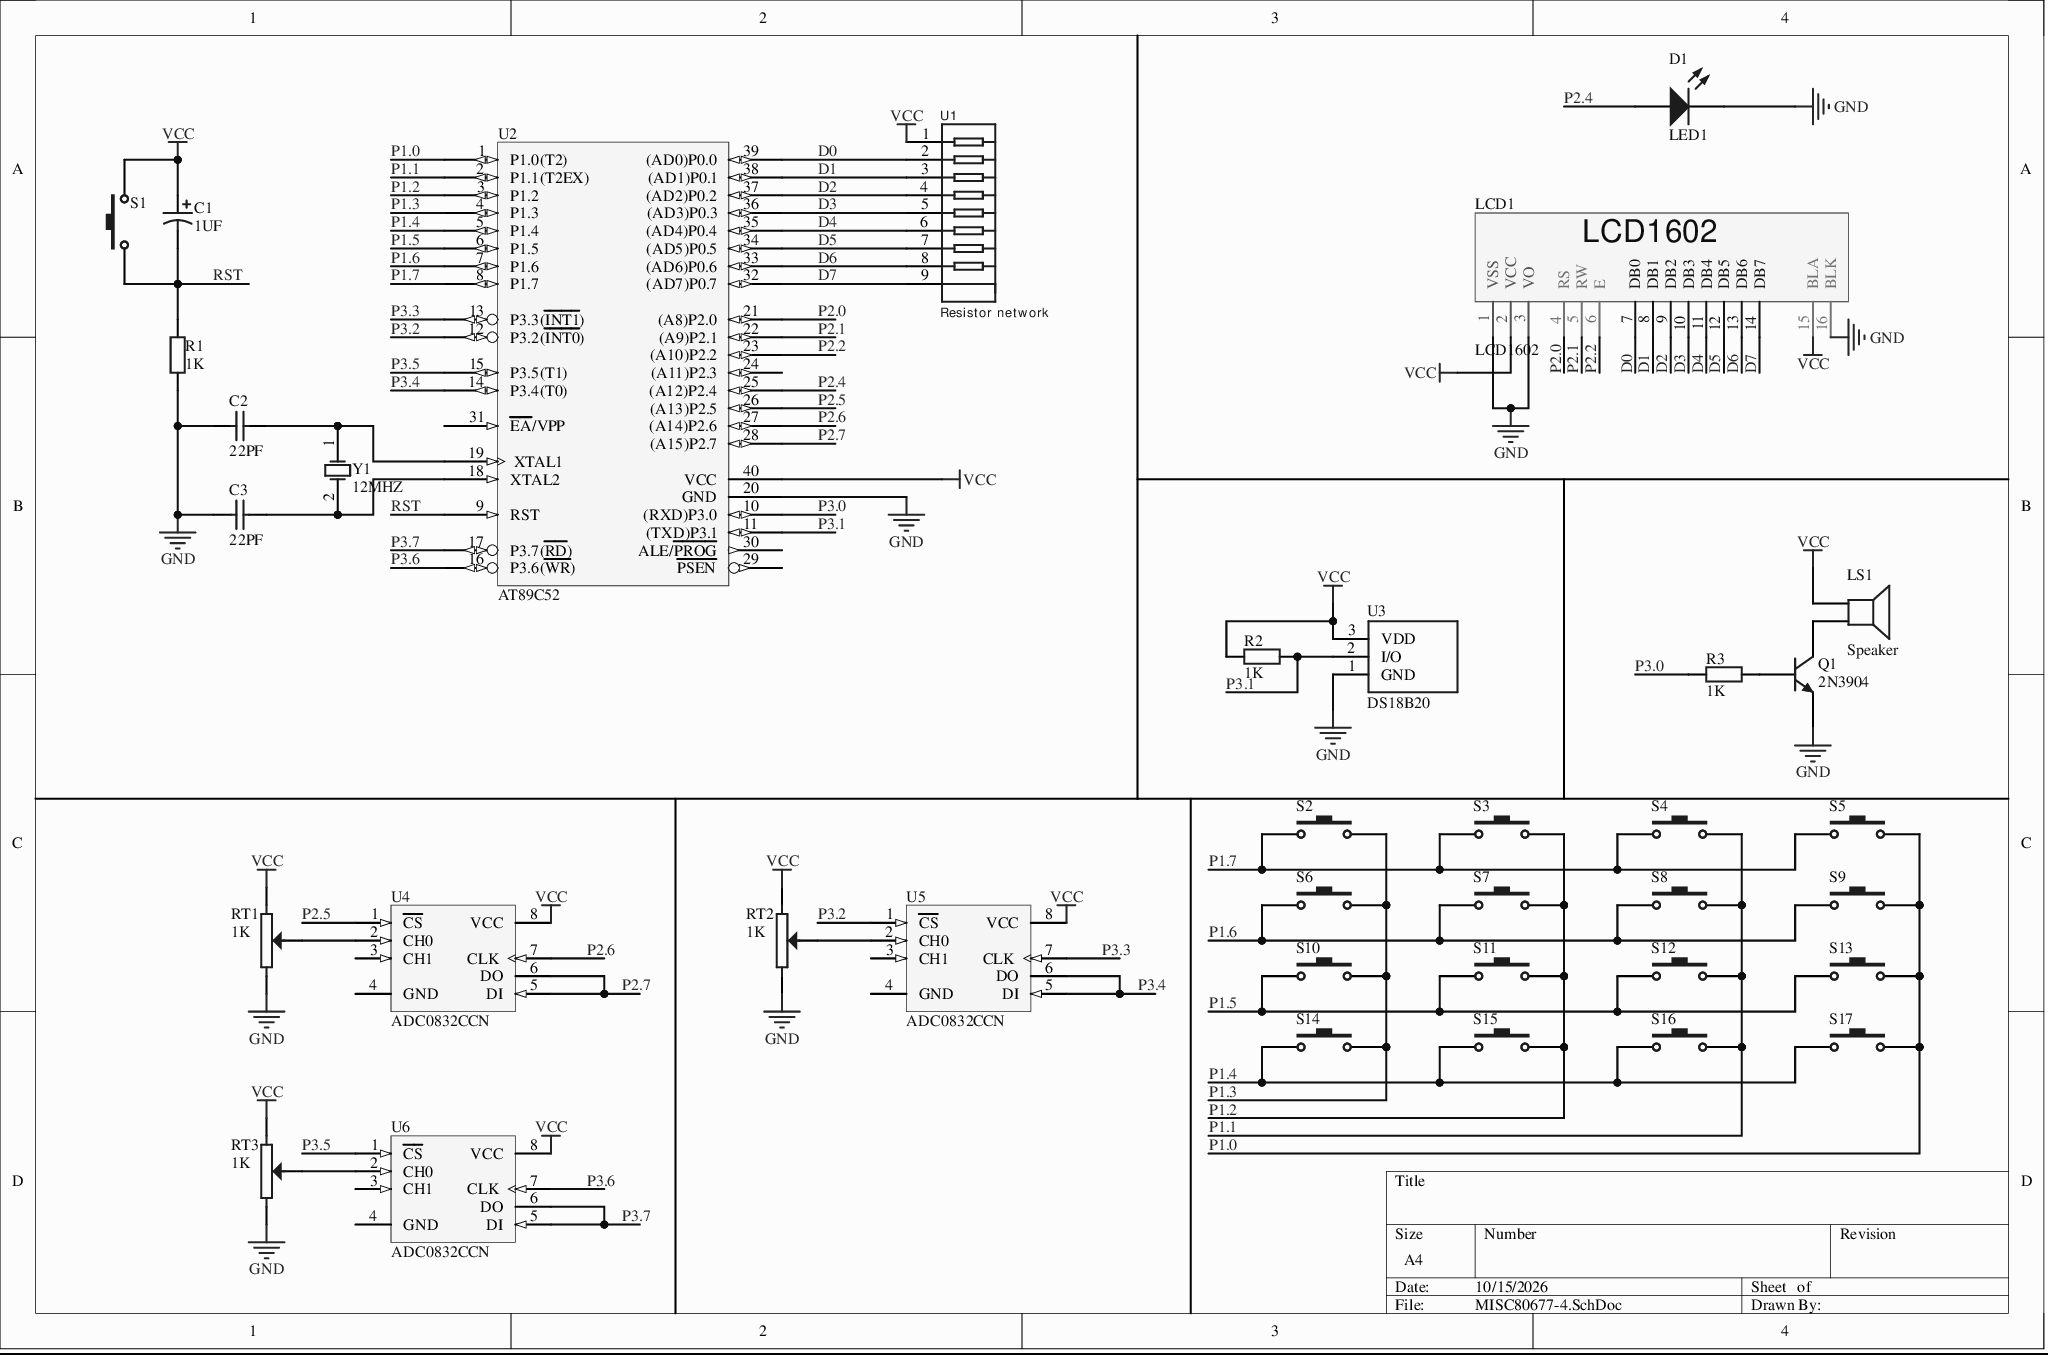
[diagram p0: MISC80677-4.SchDoc]
# Altium project MISC80677-7.PrjPcb
1 sheet, 37 parts. Net scope: global (net labels, ports and power ports of the same name join across sheets).
Board file: MISC80677.PcbDoc

## Sheet MISC80677-4.SchDoc
size A4

### Parts
C1  1UF  [RB7.6-15]
C2  22PF  [RAD-0.3]
C3  22PF  [RAD-0.3]
D1  LED1  [LED-1]
LCD1  LCD1602  [LCD1602]
LS1  Speaker  [PIN2]
Q1  2N3904  [TO-92A]
R1  1K  [AXIAL-0.4]
R2  1K  [AXIAL-0.4]
R3  1K  [AXIAL-0.4]
RT1  1K  [电位器]
RT2  1K  [电位器]
RT3  1K  [电位器]
S1  SW-PB  [SPST-2]  (value not drawn)
S2  SW-PB  [SPST-2]  (value not drawn)
S3  SW-PB  [SPST-2]  (value not drawn)
S4  SW-PB  [SPST-2]  (value not drawn)
S5  SW-PB  [SPST-2]  (value not drawn)
S6  SW-PB  [SPST-2]  (value not drawn)
S7  SW-PB  [SPST-2]  (value not drawn)
S8  SW-PB  [SPST-2]  (value not drawn)
S9  SW-PB  [SPST-2]  (value not drawn)
S10  SW-PB  [SPST-2]  (value not drawn)
S11  SW-PB  [SPST-2]  (value not drawn)
S12  SW-PB  [SPST-2]  (value not drawn)
S13  SW-PB  [SPST-2]  (value not drawn)
S14  SW-PB  [SPST-2]  (value not drawn)
S15  SW-PB  [SPST-2]  (value not drawn)
S16  SW-PB  [SPST-2]  (value not drawn)
S17  SW-PB  [SPST-2]  (value not drawn)
U1  Resistor network  [paizu]
U2  AT89C52  [DIP40]
U3  DS18B20  [DS18B20]
U4  ADC0832CCN  [N08E]
U5  ADC0832CCN  [N08E]
U6  ADC0832CCN  [N08E]
Y1  12MHZ  [R38]

### Nets
GND: C2.1 C3.1 D1.2(K) LCD1.1(VSS) LCD1.3(VO) LCD1.16(BLK) Q1.1(E) R1.1 RT1.2 RT2.2 RT3.2 U2.20(GND) U3.1(GND)
VCC: C1.1 LCD1.2(VCC) LCD1.15(BLA) LS1.1 R2.1 RT1.1 RT2.1 RT3.1 S1.2 U1.1 U2.40(VCC) U3.3(VDD) U4.8(VCC) U5.8(VCC) U6.8(VCC)
D0: LCD1.7(DB0) U1.2 U2.39((AD0)P0.0)
D1: LCD1.8(DB1) U1.3 U2.38((AD1)P0.1)
D2: LCD1.9(DB2) U1.4 U2.37((AD2)P0.2)
D3: LCD1.10(DB3) U1.5 U2.36((AD3)P0.3)
D4: LCD1.11(DB4) U1.6 U2.35((AD4)P0.4)
D5: LCD1.12(DB5) U1.7 U2.34((AD5)P0.5)
D6: LCD1.13(DB6) U1.8 U2.33((AD6)P0.6)
D7: LCD1.14(DB7) U1.9 U2.32((AD7)P0.7)
P1.0: S5.2 S9.2 S13.2 S17.2 U2.1(P1.0(T2))
P1.1: S4.2 S8.2 S12.2 S16.2 U2.2(P1.1(T2EX))
P1.2: S3.2 S7.2 S11.2 S15.2 U2.3(P1.2)
P1.3: S2.2 S6.2 S10.2 S14.2 U2.4(P1.3)
P1.4: S14.1 S15.1 S16.1 S17.1 U2.5(P1.4)
P1.5: S10.1 S11.1 S12.1 S13.1 U2.6(P1.5)
P1.6: S6.1 S7.1 S8.1 S9.1 U2.7(P1.6)
P1.7: S2.1 S3.1 S4.1 S5.1 U2.8(P1.7)
P2.0: LCD1.4(RS) U2.21((A8)P2.0)
P2.1: LCD1.5(RW) U2.22((A9)P2.1)
P2.2: LCD1.6(E) U2.23((A10)P2.2)
P2.4: D1.1(A) U2.25((A12)P2.4)
P2.5: U2.26((A13)P2.5) U4.1(~{CS})
P2.6: U2.27((A14)P2.6) U4.7(CLK)
P2.7: U2.28((A15)P2.7) U4.5(DI) U4.6(DO)
P3.0: R3.1 U2.10((RXD)P3.0)
P3.1: R2.2 U2.11((TXD)P3.1) U3.2(I/O)
P3.2: U2.12(P3.2(~{INT0})) U5.1(~{CS})
P3.3: U2.13(P3.3(~{INT1})) U5.7(CLK)
P3.4: U2.14(P3.4(T0)) U5.5(DI) U5.6(DO)
P3.5: U2.15(P3.5(T1)) U6.1(~{CS})
P3.6: U2.16(P3.6(~{WR})) U6.7(CLK)
P3.7: U2.17(P3.7(~{RD})) U6.5(DI) U6.6(DO)
RST: C1.2 R1.2 S1.1 U2.9(RST)
NetC2_2: C2.2 U2.19(XTAL1) Y1.1(OSC1)
NetC3_2: C3.2 U2.18(XTAL2) Y1.2(OSC2)
NetLS1_2: LS1.2 Q1.3(C)
NetQ1_2: Q1.2(B) R3.2
NetRT1_3: RT1.3(W) U4.2(CH0)
NetRT2_3: RT2.3(W) U5.2(CH0)
NetRT3_3: RT3.3(W) U6.2(CH0)

Not connected (* = marked no-connect by the designer): U2 24((A11)P2.3) 29(~{PSEN}) 30(ALE/~{PROG}) 31(~{EA}/VPP); U4 3(CH1) 4(GND); U5 3(CH1) 4(GND); U6 3(CH1) 4(GND)

### Library data of the parts
C1 = Cap Pol1: Polarized Capacitor (Radial); Value: 100pF; Published: 8-Jun-2000; LatestRevisionDate: 17-Jul-2002; LatestRevisionNote: Re-released for DXP Platform.; PackageReference: RB7.6-15; PackageDescription: Polarized Capacitor (Radial); 2 Leads; Publisher: Altium Limited
C2 C3 = Cap: Capacitor; Value: 100pF; Published: 8-Jun-2000; LatestRevisionDate: 17-Jul-2002; LatestRevisionNote: Re-released for DXP Platform.; PackageReference: RAD-0.3; PackageDescription: Radial Cap, Thru-Hole; 2 Leads; 0.3 in Pin Spacing; Publisher: Altium Limited
D1 = LED1: Typical RED GaAs LED; Published: 8-Jun-2000; LatestRevisionDate: 08-Jul-2005; LatestRevisionNote: Mech Layer 1 removed.; PackageReference: LED-1; PackageDescription: LED; 2 Leads; Publisher: Altium Limited
LS1 = Speaker: Loudspeaker; Published: 24-Mar-1999; LatestRevisionDate: 17-Jul-2002; LatestRevisionNote: Re-released for DXP Platform.; PackageReference: PIN2; Publisher: Altium Limited
Q1 = 2N3904: NPN General Purpose Amplifier; Published: 8-Jun-2000; LatestRevisionDate: 15-Jan-2003; LatestRevisionNote: PCB Footprint 'BCY-W3/D4.7' replaced; DatasheetVersion: 1997; PackageVersion: Sep-1998; PackageReference: TO-92A; PackageDescription: TO, Flat Index; 3 In-Line, Axial Leads; Body Dia. 4.5mm; Leads 0.51 x 0.48 mm (max); ComponentLink1Description: Manufacturer Link; ComponentLink2Description: Datasheet; ComponentLink2URL: http://www.fairchildsemi.com/ds/2N%2F2N3904.pdf; Publisher: Altium Limited
R1-R3 = Res2: Resistor; Published: 8-Jun-2000; LatestRevisionDate: 17-Jul-2002; LatestRevisionNote: Re-released for DXP Platform.; PackageReference: AXIAL-0.4; PackageDescription: Axial Device, Thru-Hole; 2 Leads; 0.4 in Pin Spacing; Value: 1K; Publisher: Altium Limited
RT1-RT3 = 电位器
S1-S17 = SW-PB: Switch; Published: 24-Mar-1999; LatestRevisionDate: 17-Jul-2002; LatestRevisionNote: Re-released for DXP Platform.; PackageReference: SPST-2; PackageDescription: Switch; 2 Leads; Publisher: Altium Limited
U1 = 排阻
U2 = STC89C52
U4-U6 = ADC0832CCN: 8-Bit Serial I/O A/D Converter with Multiplexer Option; Package Information: Latest Revision: Sep-1997; Published: 15-Apr-2002; Datasheet: Latest Revision: Aug-1999; Package Reference: N08E; Publisher: Altium Limited
Y1 = XTAL: Crystal Oscillator; Published: 8-Jun-2000; LatestRevisionDate: 17-Jul-2002; LatestRevisionNote: Re-released for DXP Platform.; PackageReference: R38; PackageDescription: Crystal, Thru-Hole; 2 Leads; Body 3.1 x 8.2 mm (Dia.xH); Publisher: Altium Limited